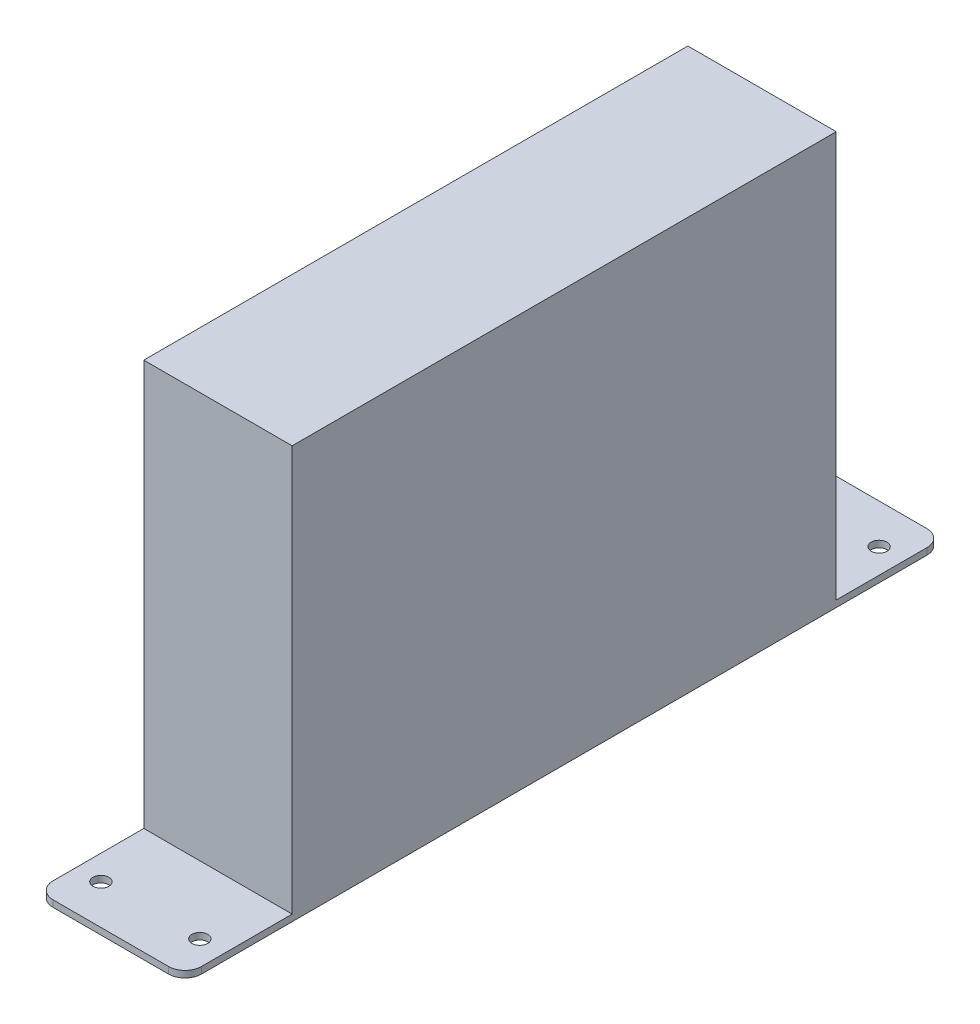
SolidWorks part; units mm, degrees
material "标准件"
ref_plane "前视基准面" through (0, 0, 0) normal (0, 0, 1) x (1, 0, 0)
ref_plane "上视基准面" through (0, 0, 0) normal (0, 1, 0) x (1, 0, 0)
ref_plane "右视基准面" through (0, 0, 0) normal (1, 0, 0) x (0, 0, -1)
sketch "草图1" plane through (0, 0, 0) normal (0, 1, 0) x (1, 0, 0)
  line L1 (-22.5, -82.5) -> (22.5, -82.5)
  line L2 (-22.5, -82.5) -> (-22.5, 82.5)
  line L3 (-22.5, 82.5) -> (22.5, 82.5)
  line L4 (22.5, -82.5) -> (22.5, 82.5)
  line L5 (-22.5, -82.5) -> (22.5, 82.5) construction
  line L6 (-22.5, 82.5) -> (22.5, -82.5) construction
  point P0 (0, 0)
  dimension "D1" = 45
  dimension "D2" = 165
extrude "凸台-拉伸1" add sketch "草图1" along normal blind 125
sketch "草图3" plane through (0, 0, 0) normal (0, 1, 0) x (1, 0, 0)
  line L0 (0, 0) -> (58.9612, 0) construction
  line L1 (-22.5, 82.5) -> (22.5, 82.5)
  line L2 (-22.5, 82.5) -> (-22.5, 115)
  line L3 (-22.5, 115) -> (22.5, 115)
  line L4 (22.5, 82.5) -> (22.5, 115)
  line L5 (22.5, -82.5) -> (22.5, -115)
  line L6 (-22.5, -115) -> (22.5, -115)
  line L7 (-22.5, -82.5) -> (-22.5, -115)
  line L8 (-22.5, -82.5) -> (22.5, -82.5)
  dimension "D1" = 230
extrude "凸台-拉伸2" add sketch "草图3" along normal blind 2
hole_wizard "M4 间隙孔1" positions "草图4" profile "草图5" hole size "M4" standard "ISO" end condition through all
sketch "草图4" plane through (0, 2, 0) normal (0, 1, 0) x (1, 0, 0)
  line L0 (0, 0) -> (0, 115) construction
  line L1 (22.5, 115) -> (-22.5, 115) construction
  line L3 (0, 0) -> (43.828, 0) construction
  point P0 (-15, 103)
  point P2 (15, 103)
  point P16 (15, -103)
  point P17 (-15, -103)
  dimension "D1" = 30
  dimension "D2" = 206
sketch "草图5" plane through (-15, 2, -103) normal (1, 0, 0) x (0, 0, 1)
  line L0 (0, 0) -> (0, 2)
  line L1 (0, 2) -> (2.4, 2)
  line L2 (2.4, 2) -> (2.4, 0)
  line L5 (2.4, 0) -> (0, 0)
  line L11 (0, -6.35) -> (0, 107.95) construction
  dimension "通孔孔直径" = 4.8
  dimension "通孔孔深度" = 2
fillet "圆角1" radius 5 4 edges at (-22.5, 1, 115) (22.5, 1, 115) (22.5, 1, -115) (-22.5, 1, -115)
